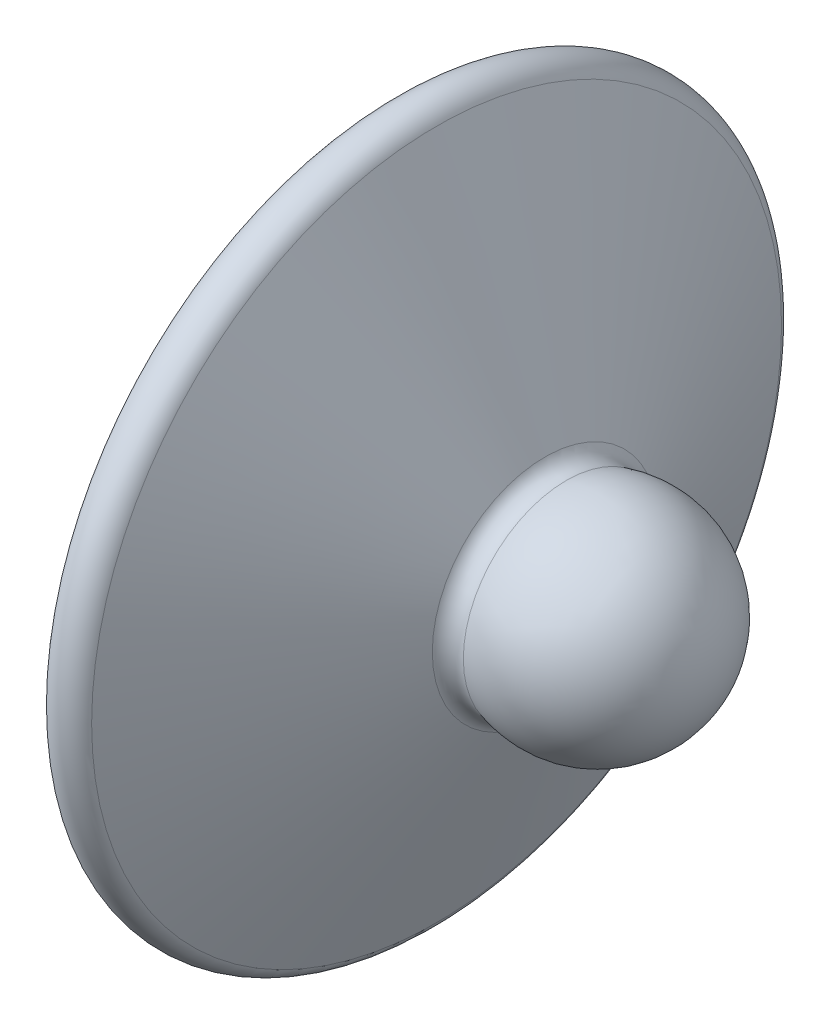
from build123d import *

# Parameters (mm, degrees)
CHAMFER1_SIZE = 1


with BuildPart() as part:
    # Sketch1 → Revolve1 (revolve)
    with BuildSketch(Plane.XY, mode=Mode.PRIVATE) as revolve1_sk:
        with BuildLine():
            Line((0, 0), (0, 6))
            Line((0, 6), (5, 6))
            Line((5, 6), (5, 18.672111461))
            ThreePointArc((5, 18.672111461), (6.040480856, 19.96852374), (7.531364262, 19.233301407))
            Line((7.531364262, 19.233301407), (13.572014794, 6.279084538))
            ThreePointArc((13.572014794, 6.279084538), (14.069886887, 5.788915703), (14.767133641, 5.744316685))
            ThreePointArc((14.767133641, 5.744316685), (20.077904543, 4.816492404), (22.5, 0))
            Line((22.5, 0), (0, 0))
        make_face()
    revolve(revolve1_sk.sketch.rotate(Axis((0, 0, 0), (1, 0, 0)), 90), axis=Axis((0, 0, 0), (1, 0, 0)))

    # Chamfer1
    chamfer1_edges = [part.edges().sort_by_distance(p)[0] for p in [
        (0, 0, -6),
    ]]
    chamfer(chamfer1_edges, length=CHAMFER1_SIZE)


solid = part.part
